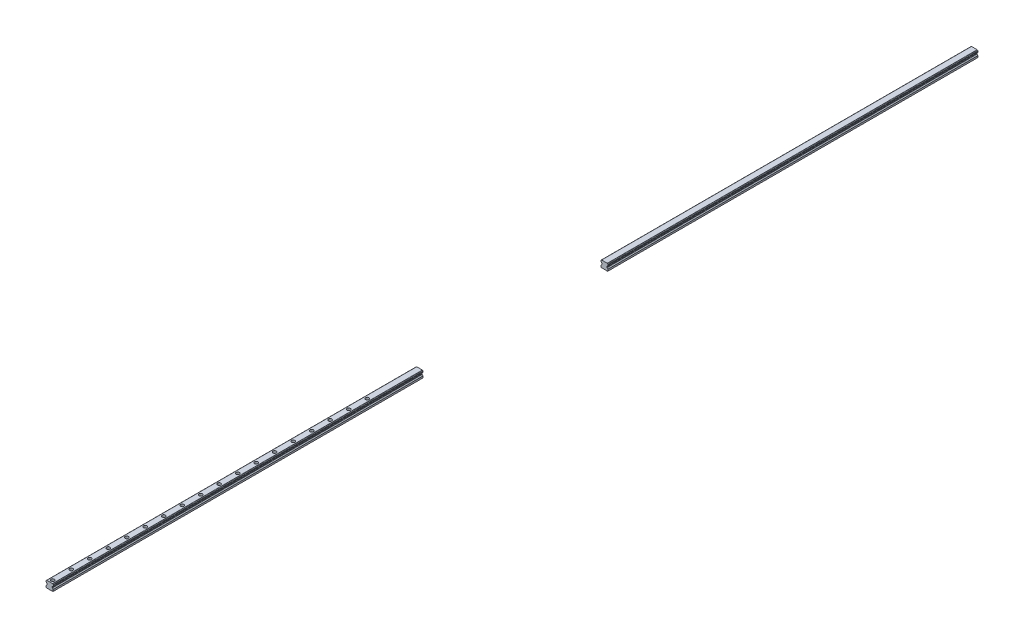
SolidWorks part; units mm, degrees
material "Q235"
ref_plane "Front Plane" through (0, 0, 0) normal (0, 0, 1) x (1, 0, 0)
ref_plane "Top Plane" through (0, 0, 0) normal (0, 1, 0) x (1, 0, 0)
ref_plane "Right Plane" through (0, 0, 0) normal (1, 0, 0) x (0, 0, -1)
sketch "Sketch1" plane through (0, 0, 0) normal (0, 1, 0) x (1, 0, 0)
  line L1 (0, -48.5) -> (0, 48.5) construction
  line L2 (-24, -35.7) -> (24, -35.7)
  line L3 (-24, -35.7) -> (-24, 35.7)
  line L4 (-24, 35.7) -> (24, 35.7)
  line L5 (24, -35.7) -> (24, 35.7)
  line L6 (-24, 0) -> (24, 0) construction
  line L7 (24, -35.7) -> (24, -42) construction
  line L8 (0, -48.5) -> (0, -60.5) construction
  line L9 (24, 35.7) -> (24, 42) construction
  point P9 (-20, 20)
  point P12 (20, 20)
  point P13 (20, -20)
  point P14 (-20, -20)
  dimension "W" = 48
  dimension "L1" = 71.4
  dimension "L0" = 97
  dimension "B" = 40
  dimension "C" = 40
  dimension "K" = 6.5
  dimension "L2" = 12
sketch "Sketch2" plane through (0, 0, 0) normal (0, 0, 1) x (1, 0, 0)
  line L0 (-24, 0) -> (24, 0) construction
  line L1 (-24, 0) -> (24, 0)
  line L2 (-24, 0) -> (-24, 33.5)
  line L3 (-24, 33.5) -> (24, 33.5)
  line L4 (24, 0) -> (24, 33.5)
  line L5 (0, 0) -> (0, 33.5) construction
  line L7 (-11.5, -6.5) -> (11.5, -6.5)
  line L8 (-24, 29.6) -> (24, 29.6)
  line L9 (-11.5, -6.5) -> (-11.5, 0)
  line L10 (-11.5, 0) -> (-8.7388, 2.7612)
  line L11 (-8.3092, 3.7983) -> (-8.3092, 5.7929)
  line L12 (-8.7388, 6.83) -> (-11.5, 9.5912)
  line L13 (-11.9296, 10.6283) -> (-11.9296, 12.6229)
  line L14 (-11.5, 13.66) -> (-10.0896, 15.0704)
  line L15 (-9.0525, 15.5) -> (9.0525, 15.5)
  line L16 (11.9296, 10.6283) -> (11.9296, 12.6229)
  line L17 (8.7388, 6.83) -> (11.5, 9.5912)
  line L18 (8.3092, 3.7983) -> (8.3092, 5.7929)
  line L19 (11.5, 0) -> (8.7388, 2.7612)
  line L20 (11.5, 13.66) -> (10.0896, 15.0704)
  line L21 (11.5, -6.5) -> (11.5, 0)
  line L22 (-11.5, -6.5) -> (-24, -6.5) construction
  arc A0 (-8.7388, 2.7612) -> (-8.3092, 3.7983) centre (-9.7759, 3.7983) ccw
  arc A1 (-8.7388, 6.83) -> (-8.3092, 5.7929) centre (-9.7759, 5.7929) cw
  arc A2 (-11.9296, 10.6283) -> (-11.5, 9.5912) centre (-10.4629, 10.6283) ccw
  arc A3 (-11.9296, 12.6229) -> (-11.5, 13.66) centre (-10.4629, 12.6229) cw
  arc A4 (-10.0896, 15.0704) -> (-9.0525, 15.5) centre (-9.0525, 14.0333) cw
  arc A5 (11.9296, 12.6229) -> (11.5, 13.66) centre (10.4629, 12.6229) ccw
  arc A6 (11.9296, 10.6283) -> (11.5, 9.5912) centre (10.4629, 10.6283) cw
  arc A7 (8.7388, 6.83) -> (8.3092, 5.7929) centre (9.7759, 5.7929) ccw
  arc A8 (8.7388, 2.7612) -> (8.3092, 3.7983) centre (9.7759, 3.7983) cw
  arc A9 (10.0896, 15.0704) -> (9.0525, 15.5) centre (9.0525, 14.0333) ccw
  circle A10 centre (24, 23.5) radius 1.65
  point P9 (-24, 21.8)
  point P33 (-9.66, 15.5)
  point P50 (0, 15.5)
  dimension "D6" = 1.4667
  dimension "(d1)" = 3.3
  dimension "D1" = 3.9
  dimension "H2" = 6.5
  dimension "H" = 40
  dimension "T" = 11.7
  dimension "D2" = 45
  dimension "W1" = 23
  dimension "D3" = 135
  dimension "H1" = 22
  dimension "D4" = 9.66
  dimension "D5" = 135
  dimension "N" = 10
  dimension "W2" = 12.5
sketch "Sketch3" plane through (0, 0, 0) normal (0, 0, 1) x (1, 0, 0)
  line L0 (-11.5, -6.5) -> (11.5, -6.5) construction
  line L1 (-11.5, -6.5) -> (-11.5, 0) construction
  line L2 (-11.5, 0) -> (-8.7388, 2.7612) construction
  line L3 (-8.3092, 3.7983) -> (-8.3092, 5.7929) construction
  line L4 (-8.7388, 6.83) -> (-11.5, 9.5912) construction
  line L5 (-11.9296, 10.6283) -> (-11.9296, 12.6229) construction
  line L6 (-11.5, 13.66) -> (-10.0896, 15.0704) construction
  line L7 (-9.0525, 15.5) -> (9.0525, 15.5) construction
  line L8 (11.5, 13.66) -> (10.0896, 15.0704) construction
  line L9 (11.9296, 10.6283) -> (11.9296, 12.6229) construction
  line L10 (8.7388, 6.83) -> (11.5, 9.5912) construction
  line L11 (8.3092, 3.7983) -> (8.3092, 5.7929) construction
  line L12 (11.5, 0) -> (8.7388, 2.7612) construction
  line L13 (11.5, -6.5) -> (11.5, 0) construction
  line L14 (-11.5, -6.5) -> (11.5, -6.5)
  line L15 (-11.5, -6.5) -> (-11.5, 0)
  line L16 (-11.5, 0) -> (-8.7388, 2.7612)
  line L17 (-8.3092, 3.7983) -> (-8.3092, 5.7929)
  line L18 (-8.7388, 6.83) -> (-11.5, 9.5912)
  line L19 (-11.9296, 10.6283) -> (-11.9296, 12.6229)
  line L20 (-11.5, 13.66) -> (-10.0896, 15.0704)
  line L21 (-9.0525, 15.5) -> (9.0525, 15.5)
  line L22 (11.5, 13.66) -> (10.0896, 15.0704)
  line L23 (11.9296, 10.6283) -> (11.9296, 12.6229)
  line L24 (8.7388, 6.83) -> (11.5, 9.5912)
  line L25 (8.3092, 3.7983) -> (8.3092, 5.7929)
  line L26 (11.5, 0) -> (8.7388, 2.7612)
  line L27 (11.5, -6.5) -> (11.5, 0)
  arc A0 (-8.7388, 2.7612) -> (-8.3092, 3.7983) centre (-9.7759, 3.7983) ccw construction
  arc A1 (-8.3092, 5.7929) -> (-8.7388, 6.83) centre (-9.7759, 5.7929) ccw construction
  arc A2 (-11.9296, 10.6283) -> (-11.5, 9.5912) centre (-10.4629, 10.6283) ccw construction
  arc A3 (-11.5, 13.66) -> (-11.9296, 12.6229) centre (-10.4629, 12.6229) ccw construction
  arc A4 (-9.0525, 15.5) -> (-10.0896, 15.0704) centre (-9.0525, 14.0333) ccw construction
  arc A5 (10.0896, 15.0704) -> (9.0525, 15.5) centre (9.0525, 14.0333) ccw construction
  arc A6 (11.9296, 12.6229) -> (11.5, 13.66) centre (10.4629, 12.6229) ccw construction
  arc A7 (11.5, 9.5912) -> (11.9296, 10.6283) centre (10.4629, 10.6283) ccw construction
  arc A8 (8.7388, 6.83) -> (8.3092, 5.7929) centre (9.7759, 5.7929) ccw construction
  arc A9 (8.3092, 3.7983) -> (8.7388, 2.7612) centre (9.7759, 3.7983) ccw construction
  arc A10 (-8.7388, 2.7612) -> (-8.3092, 3.7983) centre (-9.7759, 3.7983) ccw
  arc A11 (-8.3092, 5.7929) -> (-8.7388, 6.83) centre (-9.7759, 5.7929) ccw
  arc A12 (-11.9296, 10.6283) -> (-11.5, 9.5912) centre (-10.4629, 10.6283) ccw
  arc A13 (-11.5, 13.66) -> (-11.9296, 12.6229) centre (-10.4629, 12.6229) ccw
  arc A14 (-9.0525, 15.5) -> (-10.0896, 15.0704) centre (-9.0525, 14.0333) ccw
  arc A15 (10.0896, 15.0704) -> (9.0525, 15.5) centre (9.0525, 14.0333) ccw
  arc A16 (11.9296, 12.6229) -> (11.5, 13.66) centre (10.4629, 12.6229) ccw
  arc A17 (11.5, 9.5912) -> (11.9296, 10.6283) centre (10.4629, 10.6283) ccw
  arc A18 (8.7388, 6.83) -> (8.3092, 5.7929) centre (9.7759, 5.7929) ccw
  arc A19 (8.3092, 3.7983) -> (8.7388, 2.7612) centre (9.7759, 3.7983) ccw
extrude "Boss-Extrude1" add sketch "Sketch3" against normal blind 3000
sketch "Sketch4" plane through (0, 0, 0) normal (0, 1, 0) x (1, 0, 0)
  line L0 (0, 0) -> (0, 3000) construction
  line L1 (9.0525, 3000) -> (-9.0525, 3000) construction
  point P5 (0, 10)
  dimension "标准端距E" = 10
hole_wizard "Counterbore Hole1" positions "Sketch6" profile "Sketch5" counterbore size "M6" standard "ISO" end condition through all
sketch "Sketch6" plane through (0, 15.5, 0) normal (0, 1, 0) x (-1, 0, 0)
  point P0 (0, -10)
sketch "Sketch5" plane through (0, 15.5, -10) normal (1, 0, 0) x (0, 0, 1)
  line L0 (0, 0) -> (0, 22)
  line L1 (0, 22) -> (3.5, 22)
  line L3 (3.5, 22) -> (3.5, 9)
  line L4 (3.5, 9) -> (5.5, 9)
  line L5 (5.5, 9) -> (5.5, 0)
  line L7 (5.5, 0) -> (0, 0)
  line L11 (0, -6.35) -> (0, 107.95) construction
  dimension "(d)" = 7
  dimension "通孔孔深度" = 22
  dimension "D" = 11
  dimension "(h)" = 9
pattern_linear "LPattern1" count 18 spacing 60 along (0, 0, -1) of "Counterbore Hole1"
chamfer "Chamfer1" distance 1 angle 45 2 edges at (-11.5, -6.5, -1500) (11.5, -6.5, -1500)
sketch "Sketch7" plane through (0, 15.5, 0) normal (0, 1, 0) x (1, 0, 0)
  line L0 (9.0525, 0) -> (-9.0525, 0) construction
  line L1 (-365.0646, 1800) -> (352.2553, 1800)
  line L2 (-365.0646, 1800) -> (-365.0646, 1200)
  line L3 (-365.0646, 1200) -> (352.2553, 1200)
  line L4 (352.2553, 1800) -> (352.2553, 1200)
  line L5 (9.0525, 3000) -> (-9.0525, 3000) construction
  dimension "D1" = 1200
  dimension "D2" = 1200
extrude "Cut-Extrude1" cut sketch "Sketch7" against normal through all
